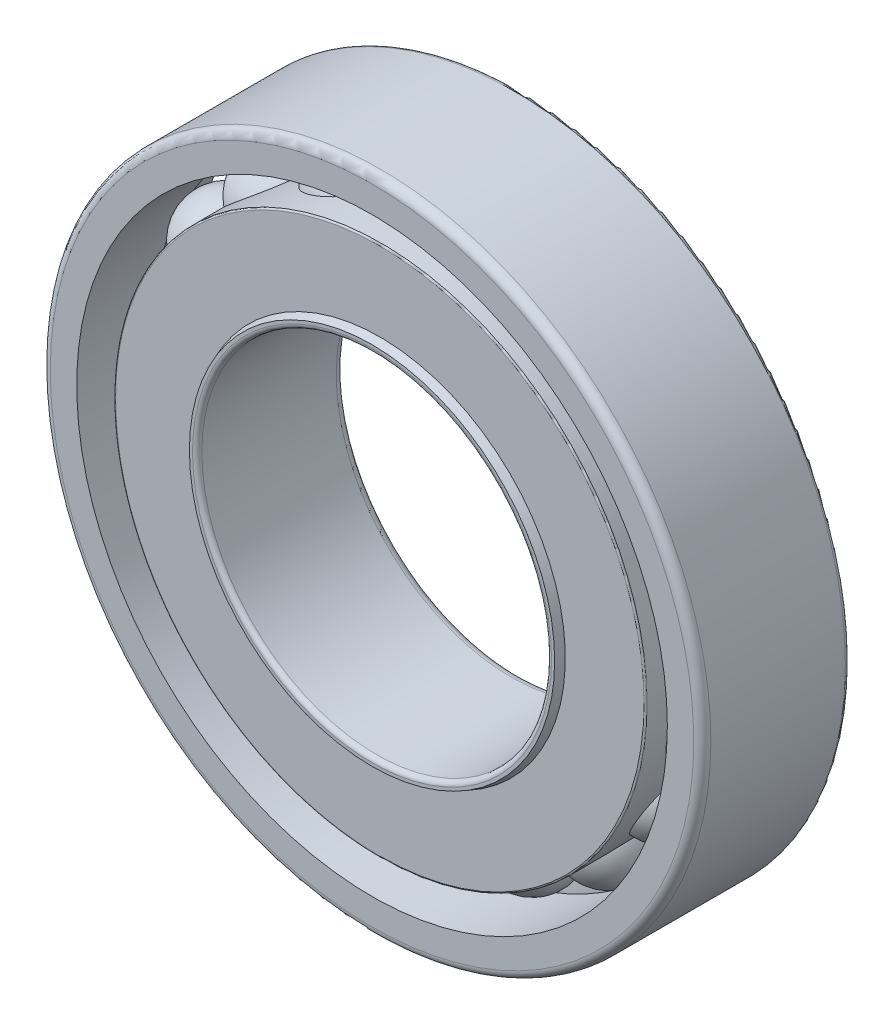
from build123d import *

# Parameters (mm, degrees)
FILLET_1_R               = 1.1
FILLET_2_R               = 0.6
PATTERN_CIRCULAR_1_COUNT = 18
SKETCH_6_W               = 7
SKETCH_6_H               = 0.3


with BuildPart() as part:
    # 草图1 → 旋转1 (revolve)
    with BuildSketch(Plane(origin=(0, 0, 0), x_dir=(0, 0, -1), z_dir=(1, 0, 0)), mode=Mode.PRIVATE) as revolve_1_sk:
        Polygon((-9.5, 38), (0, 38), (9.5, 41.5), (9.5, 42.5), (-9.5, 42.5), align=None)
    revolve(revolve_1_sk.sketch.rotate(Axis((0, 0, -50), (0, 0, 1)), 270), axis=Axis((0, 0, -50), (0, 0, 1)))

    # 草图3 → 旋转2 (revolve)
    with BuildSketch(Plane(origin=(0, 0, 0), x_dir=(0, 0, -1), z_dir=(1, 0, 0))):
        with BuildLine():
            Line((0, 38.02), (0, 26.98))
            ThreePointArc((0, 26.98), (-5.52, 32.5), (0, 38.02))
        make_face()
    revolve_2 = revolve(axis=Axis((0, 38.02, 0), (0, -1, 0)))

    # 草图2 → 旋转3 (revolve)
    with BuildSketch(Plane(origin=(0, 0, 0), x_dir=(0, 0, -1), z_dir=(1, 0, 0)), mode=Mode.PRIVATE) as revolve_3_sk:
        Polygon((-9.5, 23.5), (-9.5, 22.5), (9.5, 22.5), (9.5, 27), (0, 27), align=None)
    revolve(revolve_3_sk.sketch.rotate(Axis((0, 0, -50), (0, 0, 1)), 270), axis=Axis((0, 0, -50), (0, 0, 1)))

    # 圆角1
    fillet_1_edges = [part.edges().sort_by_distance(p)[0] for p in [
        (-22.5, 0, -9.5),
        (-42.5, 0, 9.5),
    ]]
    fillet(fillet_1_edges, radius=FILLET_1_R)

    # 圆角2
    fillet_2_edges = [part.edges().sort_by_distance(p)[0] for p in [
        (-22.5, 0, 9.5),
        (-42.5, 0, -9.5),
    ]]
    fillet(fillet_2_edges, radius=FILLET_2_R)

    # 阵列(圆周)1: 旋转2 ×18 about axis
    pattern_circular_1_axis = Axis((0, 0, 0), (0, 0, 1))
    for i in range(1, PATTERN_CIRCULAR_1_COUNT):
        add(revolve_2.rotate(pattern_circular_1_axis, i * 360 / PATTERN_CIRCULAR_1_COUNT))

    # 草图5 → 旋转4 (revolve)
    with BuildSketch(Plane(origin=(0, 0, 0), x_dir=(0, 0, -1), z_dir=(1, 0, 0)), mode=Mode.PRIVATE) as revolve_4_sk:
        with BuildLine():
            Line((-8.5, 34), (-8.5, 23.868421053))
            Line((-8.5, 23.868421053), (-8.3, 23.868421053))
            Line((-8.3, 23.868421053), (-8.3, 33.9))
            ThreePointArc((-8.3, 33.9), (-8.270710678, 33.970710678), (-8.2, 34))
            Line((-8.2, 34), (-1.5, 34))
            Line((-1.5, 34), (-1.5, 34.2))
            Line((-1.5, 34.2), (-8.3, 34.2))
            ThreePointArc((-8.3, 34.2), (-8.441421356, 34.141421356), (-8.5, 34))
        make_face()
    revolve(revolve_4_sk.sketch.rotate(Axis((0, 0, -50), (0, 0, 1)), 80.908049935), axis=Axis((0, 0, -50), (0, 0, 1)))

    # 草图6 → 旋转5 (revolve)
    with BuildSketch(Plane(origin=(0, 0, 0), x_dir=(0, 0, -1), z_dir=(1, 0, 0)), mode=Mode.PRIVATE) as revolve_5_sk:
        with Locations((4.5, 33.85)):
            Rectangle(SKETCH_6_W, SKETCH_6_H)
    revolve(revolve_5_sk.sketch.rotate(Axis((0, 0, -50), (0, 0, 1)), 270), axis=Axis((0, 0, -50), (0, 0, 1)))


solid = part.part
